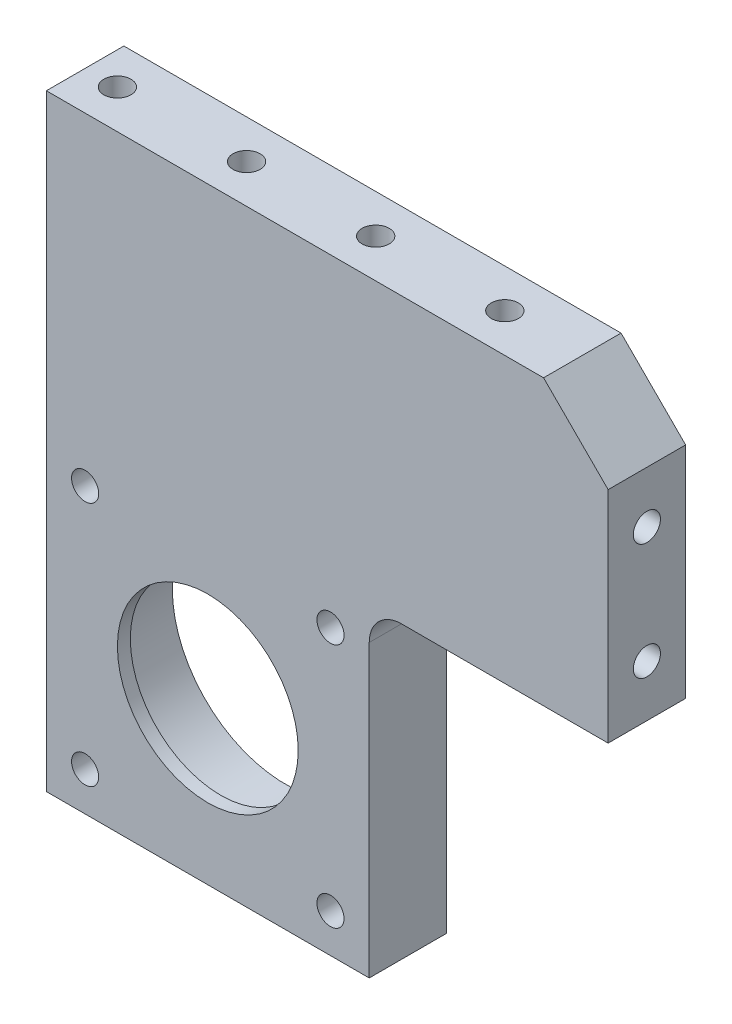
SolidWorks part; units mm, degrees
material "6061Al"
ref_plane "前视基准面" through (0, 0, 0) normal (0, 0, 1) x (1, 0, 0)
ref_plane "上视基准面" through (0, 0, 0) normal (0, 1, 0) x (1, 0, 0)
ref_plane "右视基准面" through (0, 0, 0) normal (1, 0, 0) x (0, 0, -1)
sketch "草图1" plane through (0, 0, 0) normal (0, 0, 1) x (1, 0, 0)
  line L1 (-52.5, -47.5) -> (52.5, -47.5)
  line L2 (-52.5, -47.5) -> (-52.5, 47.5)
  line L3 (-52.5, 47.5) -> (52.5, 47.5)
  line L4 (52.5, -47.5) -> (52.5, 47.5)
  line L5 (-52.5, -47.5) -> (52.5, 47.5) construction
  line L6 (-52.5, 47.5) -> (52.5, -47.5) construction
  point P0 (0, 0)
  dimension "D1" = 105
  dimension "D2" = 95
extrude "凸台-拉伸1" add sketch "草图1" along normal mid plane 12
sketch "草图10" plane through (0, 0, -6) normal (0, 0, 1) x (1, 0, 0)
  line L0 (52.5, 47.5) -> (-52.5, 47.5) construction
  line L2 (-52.5, 47.5) -> (-52.5, -47.5) construction
  circle A0 centre (-27.5, -22.5) radius 17.5
  dimension "D1" = 35
  dimension "D2" = 70
  dimension "D3" = 25
extrude "切除-拉伸1" cut sketch "草图10" along normal blind 10
sketch "草图12" plane through (0, 0, 4) normal (0, 0, -1) x (-1, 0, 0)
  circle A0 centre (27.5, -22.5) radius 14
  dimension "D1" = 28
extrude "切除-拉伸2" cut sketch "草图12" against normal through all
sketch "草图13" plane through (0, 0, 6) normal (0, 0, 1) x (1, 0, 0)
  line L0 (-52.5, -47.5) -> (52.5, -47.5) construction
  line L1 (-2.5, -47.5) -> (52.5, -47.5)
  line L2 (-2.5, -47.5) -> (-2.5, 2.5)
  line L3 (-2.5, 2.5) -> (52.5, 2.5)
  line L4 (52.5, -47.5) -> (52.5, 2.5)
  line L5 (52.5, -47.5) -> (52.5, 47.5) construction
  line L6 (-52.5, 47.5) -> (-52.5, -47.5) construction
  dimension "D1" = 50
  dimension "D2" = 50
extrude "切除-拉伸3" cut sketch "草图13" against normal through all
fillet "圆角1" radius 5 1 edges at (-2.5, 2.5, 0)
hole_wizard "M5 螺纹孔1" positions "草图14" profile "草图15" tap size "M5" standard "ISO"
sketch "草图14" plane through (0, 0, 6) normal (0, 0, 1) x (1, 0, 0)
  line L0 (-27.5, -22.5) -> (-27.5, -3.5) construction
  line L2 (-27.5, -22.5) -> (-8.5, -22.5) construction
  point P0 (-27.5, -3.5)
  point P3 (-46.5, -22.5)
  point P6 (-8.5, -22.5)
  point P9 (-27.5, -41.5)
sketch "草图15" plane through (-27.5, -3.5, 6) normal (1, 0, 0) x (0, -1, 0)
  line L0 (0, 0) -> (0, 12)
  line L1 (0, 12) -> (2.1, 12)
  line L2 (2.1, 12) -> (2.1, 0)
  line L5 (2.1, 0) -> (0, 0)
  line L11 (0, -6.35) -> (0, 107.95) construction
  dimension "通孔螺纹孔钻头直径" = 4.2
  dimension "通孔螺纹孔钻头深度" = 12
cosmetic thread "孔螺蚊线1" [suppressed] parameters "D2"=5
cosmetic thread "孔螺蚊线2" [suppressed] parameters "D2"=5
cosmetic thread "孔螺蚊线3" [suppressed] parameters "D2"=5
cosmetic thread "孔螺蚊线4" [suppressed] parameters "D2"=5
hole_wizard "M5 螺纹孔2" positions "草图16" profile "草图17" tap size "M5" standard "ISO" end condition through all
sketch "草图16" plane through (0, 0, -6) normal (0, 0, -1) x (-1, 0, 0)
  circle A0 centre (27.5, -22.5) radius 14 construction
  point P0 (8.5, -3.5)
  point P3 (8.5, -41.5)
  point P6 (46.5, -41.5)
  point P9 (46.5, -3.5)
sketch "草图17" plane through (-8.5, -3.5, -6) normal (1, 0, 0) x (0, 1, 0)
  line L0 (0, 0) -> (0, 12)
  line L1 (0, 12) -> (2.1, 12)
  line L2 (2.1, 12) -> (2.1, 0)
  line L5 (2.1, 0) -> (0, 0)
  line L11 (0, -6.35) -> (0, 107.95) construction
  dimension "通孔螺纹孔钻头直径" = 4.2
  dimension "通孔螺纹孔钻头深度" = 12
cosmetic thread "孔螺蚊线5" parameters "D2"=5
cosmetic thread "孔螺蚊线6" parameters "D2"=5
cosmetic thread "孔螺蚊线7" parameters "D2"=5
cosmetic thread "孔螺蚊线8" parameters "D2"=5
other "移动面1" face at (0, 47.5, 0) parameters "D1"=1
other "移动面2" face at (52.5, 24.5, 0) parameters "D1"=18
chamfer "倒角2" distance 10 angle 45 1 edges at (34.5, 46.5, 0)
hole_wizard "M5 螺纹孔3" positions "草图18" profile "草图19" tap size "M5" standard "ISO"
sketch "草图18" plane through (0, 46.5, 0) normal (0, 1, 0) x (1, 0, 0)
  line L1 (12.5, 0) -> (-7.5, 0) construction
  line L2 (-52.5, -6) -> (-52.5, 6) construction
  point P0 (12.5, 0)
  point P8 (-7.5, 0)
  point P9 (-27.5, 0)
  point P12 (-47.5, 0)
  dimension "D1" = 5
  dimension "D3" = 20
  dimension "D2" = 4
sketch "草图19" plane through (12.5, 46.5, 0) normal (1, 0, 0) x (0, 0, 1)
  line L0 (0, 0) -> (0, 13.6618)
  line L1 (0, 13.6618) -> (2.1, 12.4)
  line L2 (2.1, 12.4) -> (2.1, 0)
  line L5 (2.1, 0) -> (0, 0)
  line L10 (0, 13.6618) -> (-2.1, 12.4) construction
  line L11 (0, -6.35) -> (0, 107.95) construction
  dimension "螺纹孔钻头直径" = 4.2
  dimension "螺纹孔钻头深度" = 12.4
  dimension "导头角度" = 118
cosmetic thread "孔螺蚊线9" parameters "D1"=10, "D2"=5
cosmetic thread "孔螺蚊线10" parameters "D1"=10, "D2"=5
cosmetic thread "孔螺蚊线11" parameters "D1"=10, "D2"=5
cosmetic thread "孔螺蚊线14" parameters "D1"=10, "D2"=5
hole_wizard "M5 螺纹孔4" positions "草图22" profile "草图23" tap size "M5" standard "ISO"
sketch "草图22" plane through (34.5, 0, 0) normal (1, 0, 0) x (0, 0, -1)
  line L0 (0, 36.5) -> (0, 2.5) construction
  line L1 (6, 36.5) -> (-6, 36.5) construction
  line L2 (6, 2.5) -> (-6, 2.5) construction
  line L4 (-6, 46.5) -> (6, 46.5) construction
  point P0 (0, 28.5)
  point P2 (0, 10.5)
  dimension "D1" = 18
  dimension "D2" = 18
sketch "草图23" plane through (34.5, 28.5, 0) normal (0, 1, 0) x (0, 0, -1)
  line L0 (0, 0) -> (0, 13.6618)
  line L1 (0, 13.6618) -> (2.1, 12.4)
  line L2 (2.1, 12.4) -> (2.1, 0)
  line L5 (2.1, 0) -> (0, 0)
  line L10 (0, 13.6618) -> (-2.1, 12.4) construction
  line L11 (0, -6.35) -> (0, 107.95) construction
  dimension "螺纹孔钻头直径" = 4.2
  dimension "螺纹孔钻头深度" = 12.4
  dimension "导头角度" = 118
cosmetic thread "孔螺蚊线12" parameters "D1"=10, "D2"=5
cosmetic thread "孔螺蚊线13" parameters "D1"=10, "D2"=5
equation "\"D2@草图14\"=\"D1@草图14\""
equation "\"D1@草图16\"=\"D2@草图16\""
